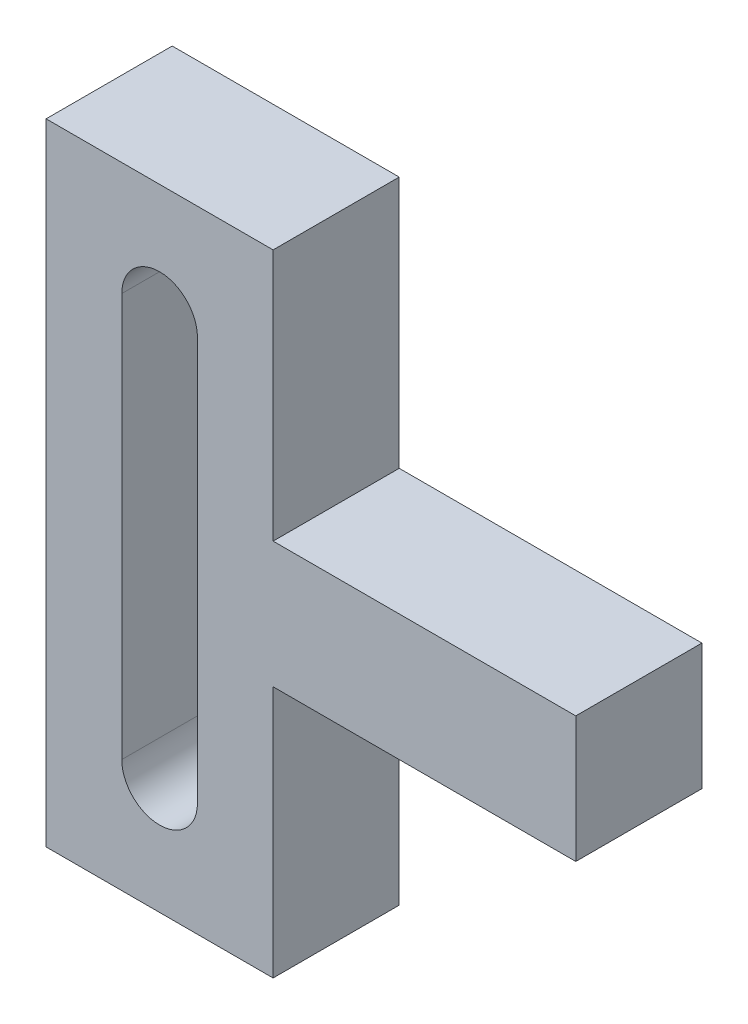
from build123d import *

# Parameters (mm, degrees)
EXTRUDE_1_DEPTH = 2.5


with BuildPart() as part:
    # 草图1 → 凸台-拉伸1 (new, symmetric)
    with BuildSketch(Plane.XY):
        Polygon((0, 0), (0, 2.5), (-12, 2.5), (-12, 12.5), (-21, 12.5), (-21, -12.5), (-12, -12.5), (-12, -2.5), (0, -2.5), align=None)
        with BuildLine():
            Line((-18, -8), (-18, 8))
            ThreePointArc((-18, 8), (-16.5, 9.5), (-15, 8))
            Line((-15, 8), (-15, -8))
            ThreePointArc((-15, -8), (-16.5, -9.5), (-18, -8))
        make_face(mode=Mode.SUBTRACT)
    extrude(amount=EXTRUDE_1_DEPTH, both=True)


solid = part.part
